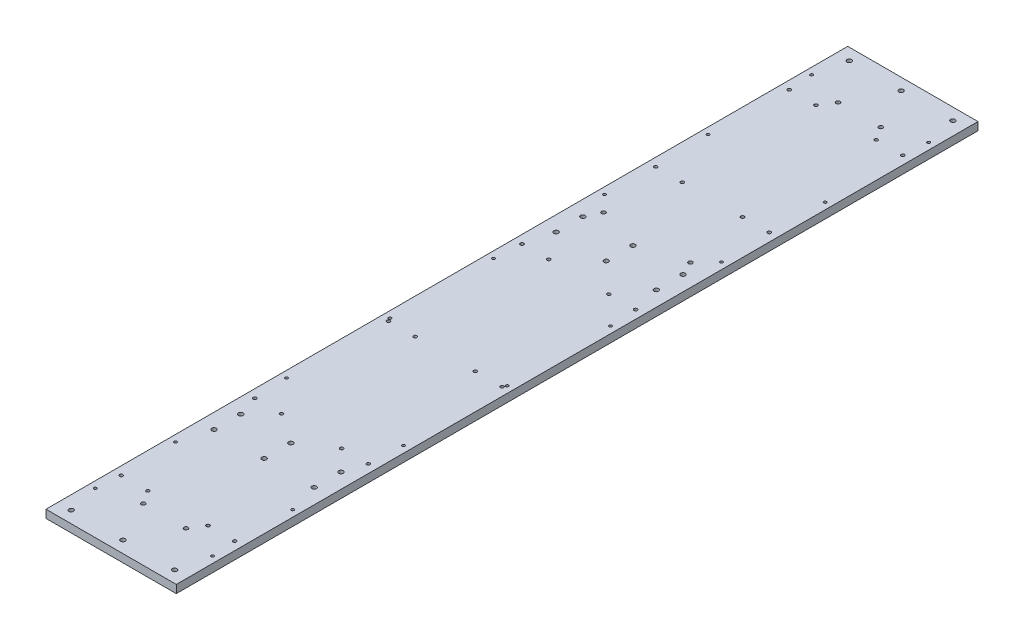
from build123d import *

# Parameters (mm, degrees)
EXTRUDE_1_DEPTH     = 600
SKETCH_2_W          = 195
SKETCH_2_H          = 38
CUT_EXTRUDE_1_DEPTH = 1205.328132197
HOLE_WIZARD_M6_1_D  = 5
HOLE_WIZARD_M8_1_D  = 6.8
F_6_0MM_1_D         = 6
HOLE_WIZARD_M5_1_D  = 4.2
HOLE_WIZARD_M8_2_D  = 6.8
F_6_0MM_2_D         = 6


with BuildPart() as part:
    # 草图1 → 凸台-拉伸1 (new, symmetric)
    with BuildSketch(Plane.XY):
        Polygon((-97.5, 30), (97.5, 30), (97.5, -20), (85.5, -20), (85.5, 18), (-85.5, 18), (-85.5, -20), (-97.5, -20), align=None)
    extrude(amount=EXTRUDE_1_DEPTH, both=True)

    # 草图2 → 切除-拉伸1 (cut, through all)
    with BuildSketch(Plane(origin=(0, 0, -600), x_dir=(-1, 0, 0), z_dir=(0, 0, -1))):
        with Locations((0, -1)):
            Rectangle(SKETCH_2_W, SKETCH_2_H)
    extrude(amount=-CUT_EXTRUDE_1_DEPTH, mode=Mode.SUBTRACT)

    # M6 螺纹孔1 (through all)
    with Locations(Plane(origin=(0, 18, 0), x_dir=(-1, 0, 0), z_dir=(0, -1, 0))):
        with Locations((45, 500), (85, 500), (45, 300), (85, 300), (45, 100), (85, 100), (45, -100), (85, -100), (45, -300), (85, -300), (45, -500), (85, -500), (-85, 500), (-45, 500), (-85, 300), (-45, 300), (-85, 100), (-45, 100), (-85, -100), (-45, -100), (-85, -300), (-45, -300), (-85, -500), (-45, -500)):
            Hole(HOLE_WIZARD_M6_1_D / 2)

    # M8 螺纹孔1 (through all)
    with Locations(Plane(origin=(0, 30, 0), x_dir=(1, 0, 0), z_dir=(0, 1, 0))):
        with Locations((-77.5, 582.3683), (0, 582.3683), (77.5, 582.3683), (-77.5, -582.3683), (0, -582.3683), (77.5, -582.3683)):
            Hole(HOLE_WIZARD_M8_1_D / 2)

    # Ø6.0mm 暗销孔1 (through all)
    with Locations(Plane(origin=(0, 18, 0), x_dir=(-1, 0, 0), z_dir=(0, -1, 0))):
        with Locations((32, 520), (-32, 520), (-32, -520), (32, -520)):
            Hole(F_6_0MM_1_D / 2)

    # M5 螺纹孔1 (through all)
    with Locations(Plane(origin=(0, 30, 0), x_dir=(1, 0, 0), z_dir=(0, 1, 0))):
        with Locations((87.6317, 536), (87.6317, 381), (87.6317, 226), (87.6317, 60), (87.6317, -95), (87.6317, -250), (87.6317, -416), (87.6317, -536), (-87.6317, -536), (-87.6317, -416), (-87.6317, -250), (-87.6317, -95), (-87.6317, 60), (-87.6317, 226), (-87.6317, 381), (-87.6317, 536)):
            Hole(HOLE_WIZARD_M5_1_D / 2)

    # M8 螺纹孔2 (through all)
    with Locations(Plane(origin=(0, 30, 0), x_dir=(1, 0, 0), z_dir=(0, 1, 0))):
        with Locations((-75, -331), (-75, -371), (0, -331), (0, -371), (75, -331), (75, -371), (-75, 181), (-75, 141), (0, 181), (0, 141), (75, 181), (75, 141)):
            Hole(HOLE_WIZARD_M8_2_D / 2)

    # Ø6.0mm 暗销孔2 (through all)
    with Locations(Plane(origin=(0, 30, 0), x_dir=(1, 0, 0), z_dir=(0, 1, 0))):
        with Locations((-65, 202), (65, 202)):
            Hole(F_6_0MM_2_D / 2)


solid = part.part
